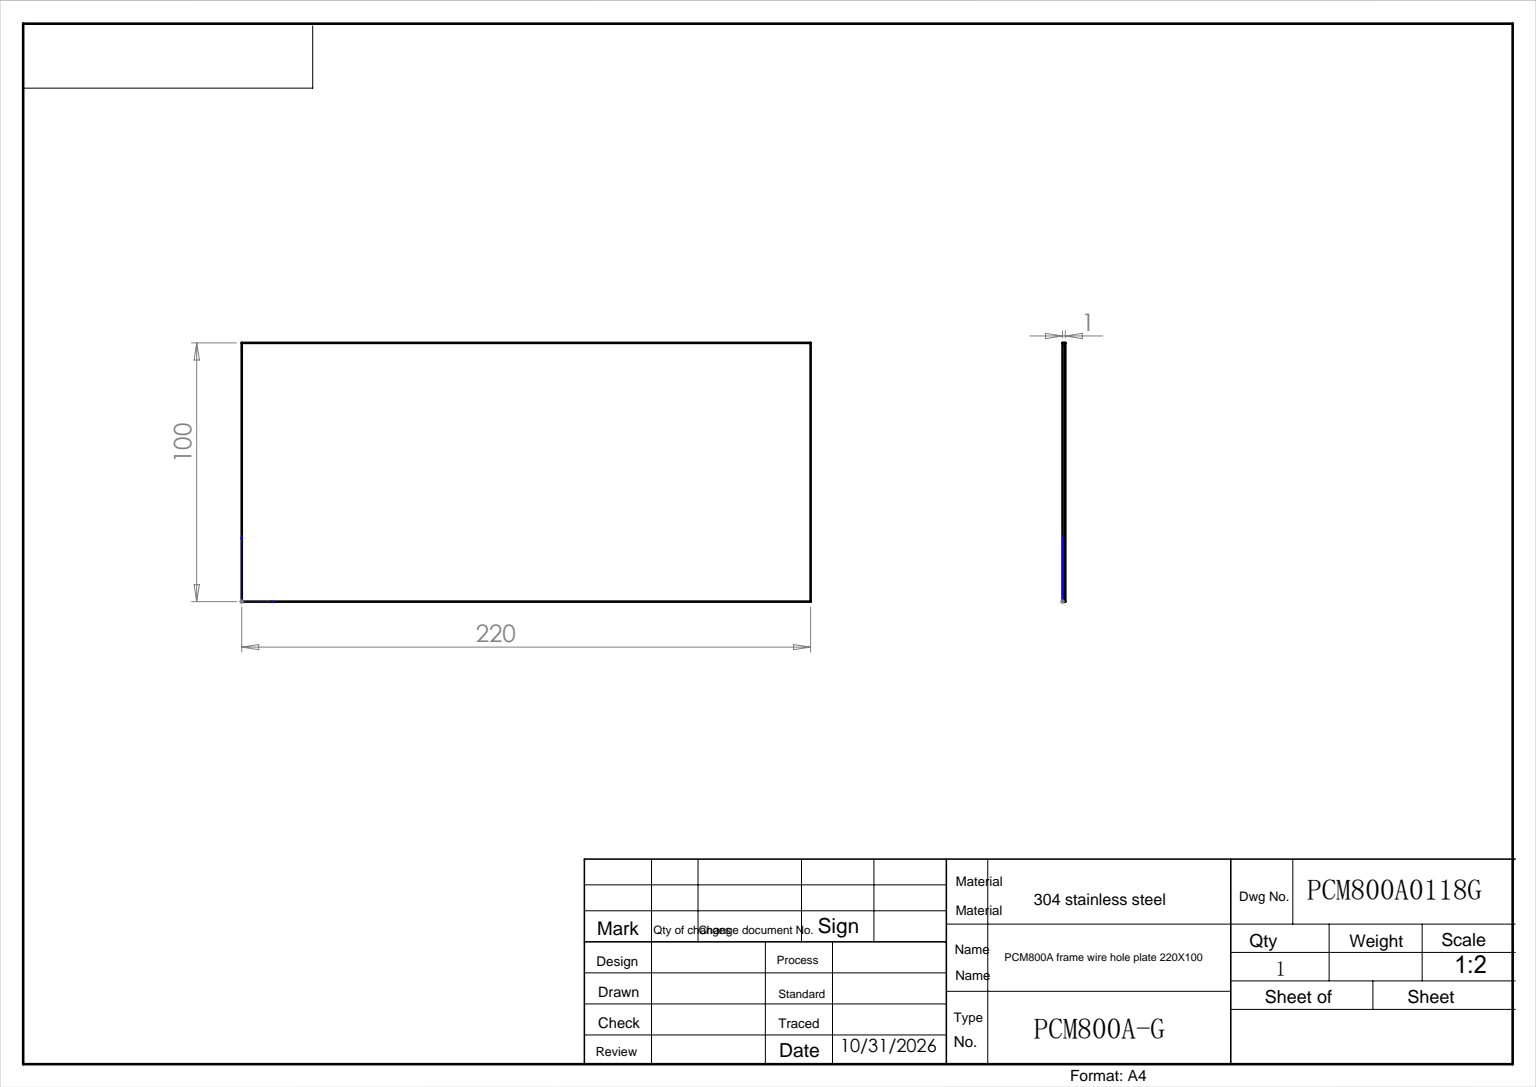
SolidWorks part; units mm, degrees
ref_plane "前视基准面" through (0, 0, 0) normal (0, 0, 1) x (1, 0, 0)
ref_plane "上视基准面" through (0, 0, 0) normal (0, 1, 0) x (1, 0, 0)
ref_plane "右视基准面" through (0, 0, 0) normal (1, 0, 0) x (0, 0, -1)
sketch "草图1" plane through (0, 0, 0) normal (0, 0, 1) x (1, 0, 0)
  line L0 (110, 100) -> (110, 22.8403) construction
  line L1 (0, 0) -> (220, 0)
  line L2 (0, 0) -> (0, 100)
  line L3 (0, 100) -> (220, 100)
  line L4 (220, 0) -> (220, 100)
  line L5 (0, 50) -> (114.8394, 50) construction
  line L6 (0, 0) -> (220, 100) construction
  dimension "D1" = 220
  dimension "D2" = 100
extrude "凸台-拉伸1" add sketch "草图1" along normal blind 1
